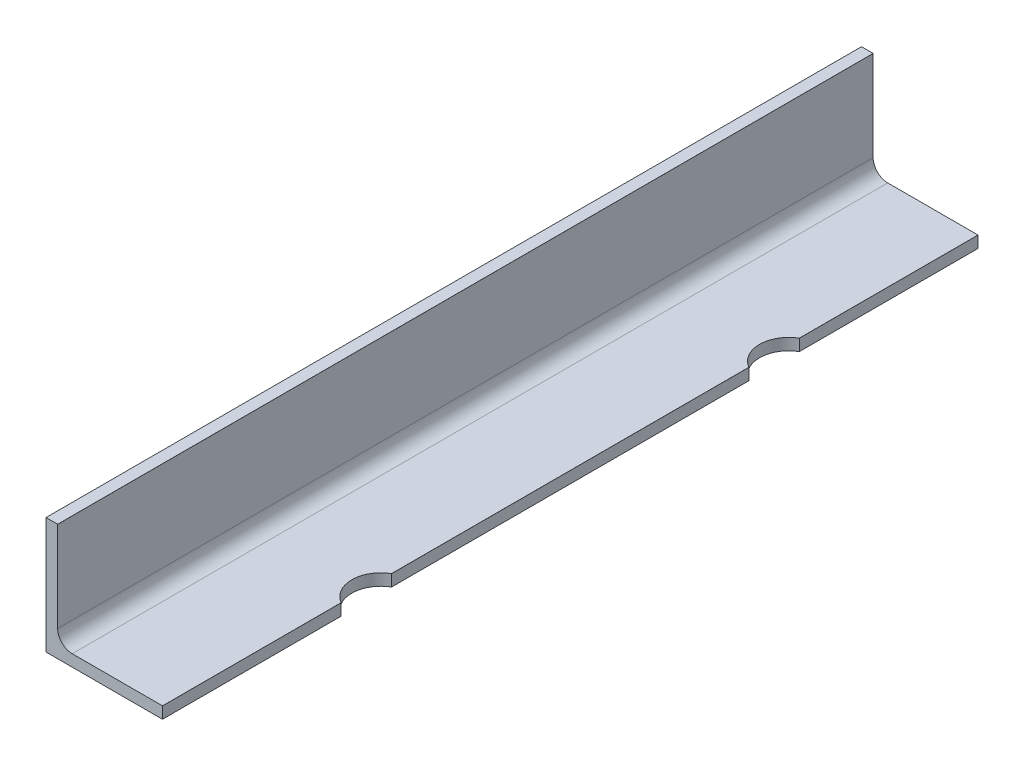
SolidWorks part; units mm, degrees
material "热轧等边角钢 Q235A"
ref_plane "前视基准面" through (0, 0, 0) normal (0, 0, 1) x (1, 0, 0)
ref_plane "上视基准面" through (0, 0, 0) normal (0, 1, 0) x (1, 0, 0)
ref_plane "右视基准面" through (0, 0, 0) normal (1, 0, 0) x (0, 0, -1)
sketch "草图1" plane through (0, 0, 0) normal (0, 0, 1) x (1, 0, 0)
  line L0 (0, 0) -> (0, 40)
  line L1 (0, 40) -> (3.99, 40)
  line L2 (4, 39.99) -> (4, 9)
  line L3 (9, 4) -> (39.99, 4)
  line L4 (40, 3.99) -> (40, 0)
  line L5 (40, 0) -> (0, 0)
  arc A0 (4, 39.99) -> (3.99, 40) centre (3.99, 39.99) ccw
  arc A1 (9, 4) -> (4, 9) centre (9, 9) cw
  arc A2 (40, 3.99) -> (39.99, 4) centre (39.99, 3.99) ccw
  point P9 (4, 40)
  point P14 (40, 4)
extrude "拉伸1" add sketch "草图1" along normal blind 280
sketch "草图2" plane through (0, 4, 0) normal (0, 1, 0) x (1, 0, 0)
  line L0 (39.99, -280) -> (9, -280) construction
  line L1 (39.99, -280) -> (39.99, 0) construction
  circle A0 centre (45, -210) radius 10
  circle A1 centre (45, -70) radius 10
  dimension "D1" = 20
  dimension "D2" = 20
  dimension "D3" = 70
  dimension "D4" = 140
  dimension "D5" = 5.01
  dimension "D6" = 5.01
extrude "切除-拉伸1" cut sketch "草图2" against normal blind 10
equation "\"D2@草图1\" = \"D1@草图1\""
equation "\"D4@草图1\" = \"D3@草图1\""
equation "\"D7@草图1\" = \"D5@草图1\""
